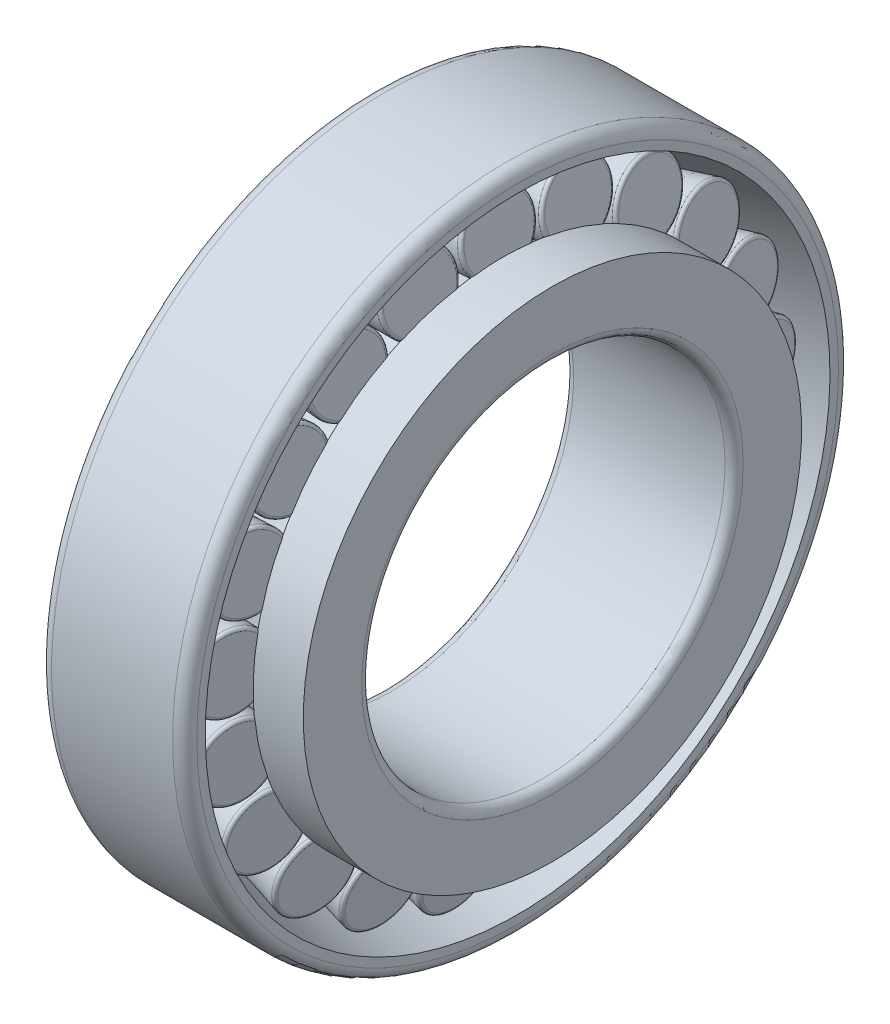
from build123d import *

# Parameters (mm, degrees)
CIRCULAR_PATTERN1_COUNT = 21


with BuildPart() as part:
    # Sketch1 → Revolve1 (revolve)
    with BuildSketch(Plane.XY):
        with BuildLine():
            Line((17.75, 41.159456812), (9.465132405, 41.159456812))
            Line((9.465132405, 41.159456812), (10, 38.159456812))
            Line((10, 38.159456812), (-7.093552866, 36.631191387))
            Line((-7.093552866, 36.631191387), (-7.360986664, 38.131191387))
            Line((-7.360986664, 38.131191387), (-10.25, 38.131191387))
            Line((-10.25, 38.131191387), (-10.25, 31.5))
            ThreePointArc((-10.25, 31.5), (-9.810660172, 30.439339828), (-8.75, 30))
            Line((-8.75, 30), (16.25, 30))
            ThreePointArc((16.25, 30), (17.310660172, 30.439339828), (17.75, 31.5))
            Line((17.75, 31.5), (17.75, 41.159456812))
        make_face()
    revolve(axis=Axis((17.75, 0, 0), (-1, 0, 0)))

    # Sketch2 → Revolve2 (revolve)
    with BuildSketch(Plane.XY):
        with BuildLine():
            Line((-7.947715946, 41.308130333), (8.922680954, 44.315939872))
            Line((8.922680954, 44.315939872), (9.92774649, 38.678663214))
            ThreePointArc((9.92774649, 38.678663214), (9.832763688, 38.287277007), (9.480034057, 38.092888985))
            Line((9.480034057, 38.092888985), (-6.653680329, 36.650438836))
            ThreePointArc((-6.653680329, 36.650438836), (-7.001831228, 36.751197373), (-7.190443516, 37.060691696))
            Line((-7.190443516, 37.060691696), (-7.947715946, 41.308130333))
        make_face()
    revolve2 = revolve(axis=Axis((-7.947715946, 41.308130333, 0), (0.9844756212878087, 0.1755213693257405, 0)))

    # Sketch3 → Revolve3 (revolve)
    with BuildSketch(Plane.XY):
        with BuildLine():
            Line((-12, 45.118), (12, 51.597741532))
            Line((12, 51.597741532), (12, 53))
            ThreePointArc((12, 53), (11.414213562, 54.414213562), (10, 55))
            Line((10, 55), (-10, 55))
            ThreePointArc((-10, 55), (-11.414213562, 54.414213562), (-12, 53))
            Line((-12, 53), (-12, 45.118))
        make_face()
    revolve(axis=Axis((17.75, 0, 0), (-1, 0, 0)))

    # Circular-Pattern1: Revolve2 ×21 about axis
    circular_pattern1_axis = Axis((0, 0, 0), (1, 0, 0))
    for i in range(1, CIRCULAR_PATTERN1_COUNT):
        add(revolve2.rotate(circular_pattern1_axis, i * 360 / CIRCULAR_PATTERN1_COUNT))


solid = part.part
